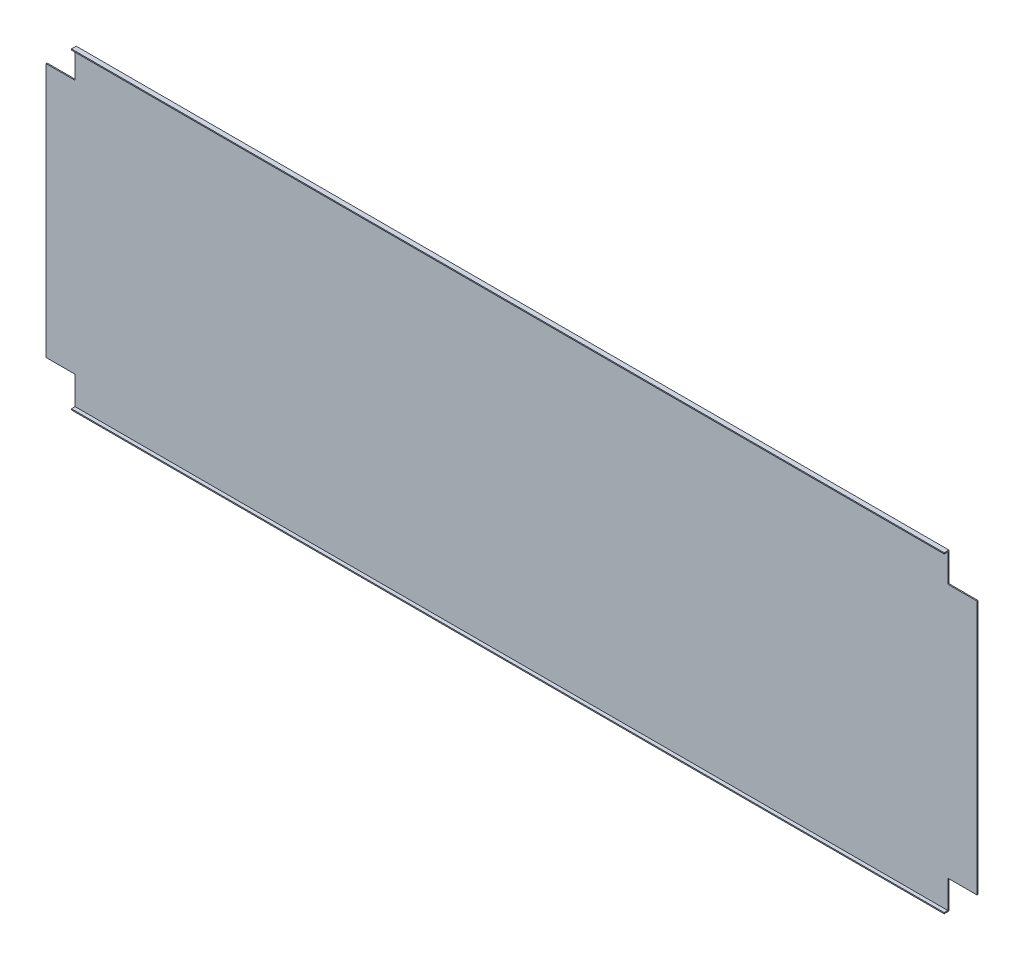
from build123d import *

# Parameters (mm, degrees)
BOSS_EXTRUDE1_DEPTH = 1.5
SKETCH2_W           = 1200
SKETCH2_H           = 1.5
BOSS_EXTRUDE2_DEPTH = 5


with BuildPart() as part:
    # Sketch1 → Boss-Extrude1 (new body)
    with BuildSketch(Plane.XY):
        Polygon((40, 0), (1240, 0), (1240, 40), (1280, 40), (1280, 390), (1240, 390), (1240, 430), (40, 430), (40, 390), (0, 390), (0, 40), (40, 40), align=None)
    extrude(amount=BOSS_EXTRUDE1_DEPTH)

    # Sketch2 → Boss-Extrude2 (add)
    with BuildSketch(Plane.XY.offset(1.5)):
        with Locations((640, 429.25)):
            Rectangle(SKETCH2_W, SKETCH2_H)
        with Locations((640, 0.75)):
            Rectangle(SKETCH2_W, SKETCH2_H)
    extrude(amount=BOSS_EXTRUDE2_DEPTH)


solid = part.part
